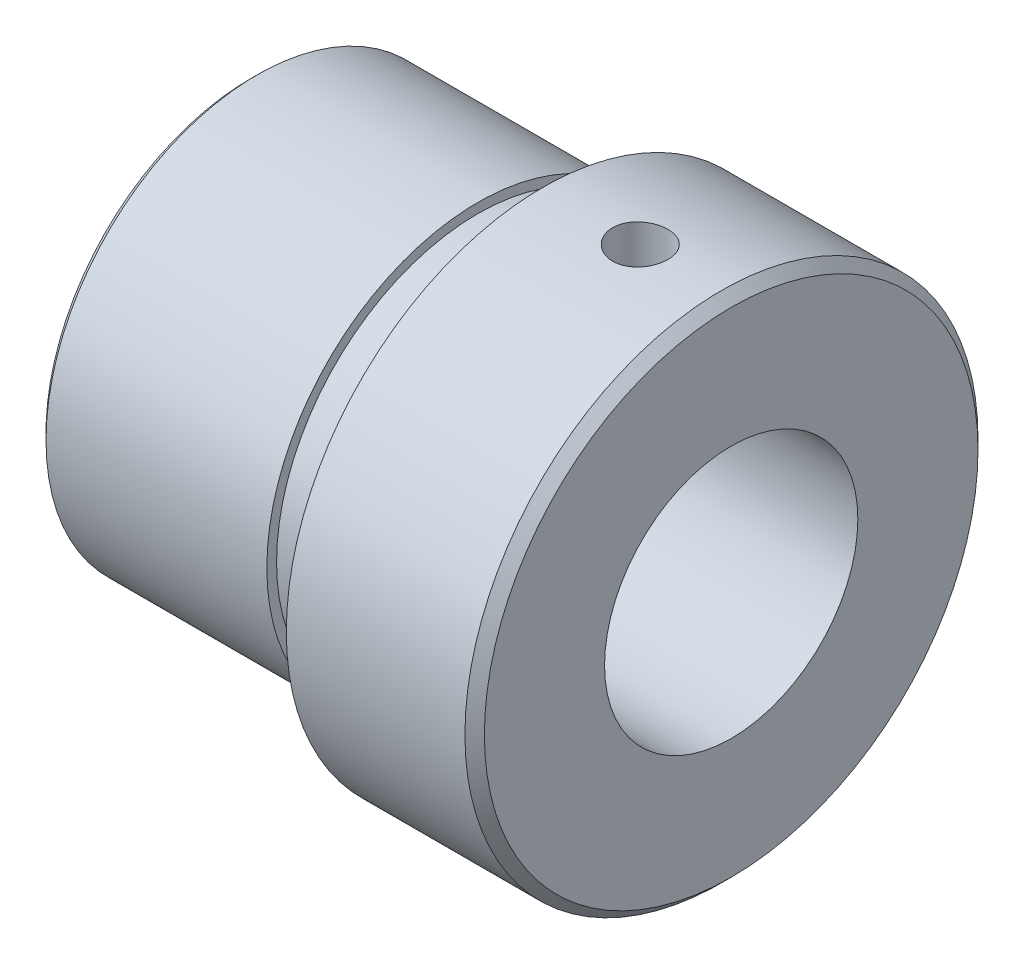
from build123d import *

# Parameters (mm, degrees)
SKETCH1_R              = 39.5
BOSS_EXTRUDE1_DEPTH    = 144
SKETCH2_OUTSIDE_W      = 117.452
SKETCH2_OUTSIDE_H      = 117.452
SKETCH2_OUTSIDE_R      = 22.5
CUT_EXTRUDE1_DEPTH     = 70
SKETCH4_OUTSIDE_W      = 117.452
SKETCH4_OUTSIDE_H      = 117.452
SKETCH4_OUTSIDE_R      = 32.5
CUT_EXTRUDE3_DEPTH     = 45
SKETCH6_OUTSIDE_W      = 117.452
SKETCH6_OUTSIDE_H      = 117.452
SKETCH6_OUTSIDE_R      = 31
CUT_EXTRUDE5_DEPTH     = 10
CHAMFER1_SIZE          = 1
CHAMFER7_SIZE          = 1.5
SKETCH12_R             = 4.25
CUT_EXTRUDE8_DEPTH     = 2
SKETCH15_R             = 63.738357407
CUT_EXTRUDE9_DEPTH     = 70
M42X3_0_TAPPED_HOLE1_D = 39


with BuildPart() as part:
    # Sketch1 → Boss-Extrude1 (new body)
    with BuildSketch(Plane(origin=(0, 0, 0), x_dir=(0, 0, -1), z_dir=(1, 0, 0))):
        Circle(SKETCH1_R)
    extrude(amount=BOSS_EXTRUDE1_DEPTH)

    # Sketch2 outside → Cut-Extrude1 (cut)
    with BuildSketch(Plane(origin=(144, 0, 0), x_dir=(0, 0, -1), z_dir=(1, 0, 0))):
        Rectangle(SKETCH2_OUTSIDE_W, SKETCH2_OUTSIDE_H)
        Circle(SKETCH2_OUTSIDE_R, mode=Mode.SUBTRACT)
    extrude(amount=-CUT_EXTRUDE1_DEPTH, mode=Mode.SUBTRACT)

    # Sketch4 outside → Cut-Extrude3 (cut)
    with BuildSketch(Plane.ZY):
        Rectangle(SKETCH4_OUTSIDE_W, SKETCH4_OUTSIDE_H)
        Circle(SKETCH4_OUTSIDE_R, mode=Mode.SUBTRACT)
    extrude(amount=-CUT_EXTRUDE3_DEPTH, mode=Mode.SUBTRACT)

    # Sketch6 outside → Cut-Extrude5 (cut)
    with BuildSketch(Plane.ZY.offset(-45)):
        Rectangle(SKETCH6_OUTSIDE_W, SKETCH6_OUTSIDE_H)
        Circle(SKETCH6_OUTSIDE_R, mode=Mode.SUBTRACT)
    extrude(amount=CUT_EXTRUDE5_DEPTH, mode=Mode.SUBTRACT)

    # Chamfer1
    chamfer1_edges = [part.edges().sort_by_distance(p)[0] for p in [
        (144, 0, 22.5),
        (0, 0, -32.5),
    ]]
    chamfer(chamfer1_edges, length=CHAMFER1_SIZE)

    # Chamfer7
    chamfer7_edges = [part.edges().sort_by_distance(p)[0] for p in [
        (74, 0, 39.5),
    ]]
    chamfer(chamfer7_edges, length=CHAMFER7_SIZE)

    # Sketch12 → Cut-Extrude8 (cut)
    with BuildSketch(Plane(origin=(0, -39.5, 0), x_dir=(-1, 0, 0), z_dir=(0, -1, 0))):
        with Locations(Location((-60, 0, 0), (0, 0, 90))):
            Circle(SKETCH12_R)
    cut_extrude8 = extrude(amount=-CUT_EXTRUDE8_DEPTH, mode=Mode.SUBTRACT)

    # Sketch14 → M10 Tapped Hole1 (revolve, cut)
    with BuildSketch(Plane(origin=(60, -37.5, 0), x_dir=(0, 0, -1), z_dir=(1, 0, 0))):
        Polygon((0, 0), (0, 12.553657631), (4.25, 10), (4.25, 0), align=None)
    m10_tapped_hole1 = revolve(axis=Axis((60, -43.85, 0), (0, 1, 0)), mode=Mode.SUBTRACT)

    # Mirror1: Cut-Extrude8, M10 Tapped Hole1 across plane
    add(cut_extrude8.mirror(Plane.ZX), mode=Mode.SUBTRACT)
    add(m10_tapped_hole1.mirror(Plane.ZX), mode=Mode.SUBTRACT)

    # Sketch15 → Cut-Extrude9 (cut)
    with BuildSketch(Plane(origin=(144, 0, 0), x_dir=(0, 0, -1), z_dir=(1, 0, 0))):
        Circle(SKETCH15_R)
    extrude(amount=-CUT_EXTRUDE9_DEPTH, mode=Mode.SUBTRACT)

    # M42x3.0 Tapped Hole1 (through all)
    with Locations(Plane(origin=(74, 0, 0), x_dir=(0, 0, -1), z_dir=(1, 0, 0))):
        with Locations((0, 0)):
            Hole(M42X3_0_TAPPED_HOLE1_D / 2)


solid = part.part
